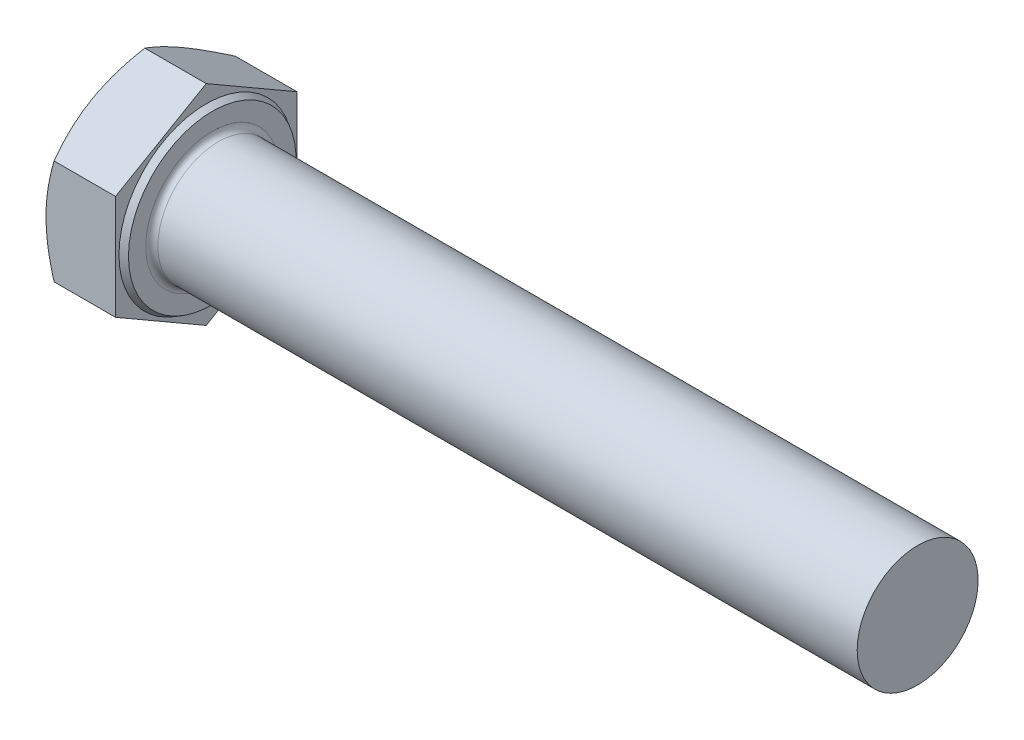
SolidWorks part; units mm, degrees
material "Q235"
ref_plane "Front Plane" through (0, 0, 0) normal (0, 0, 1) x (1, 0, 0)
ref_plane "Top Plane" through (0, 0, 0) normal (0, 1, 0) x (1, 0, 0)
ref_plane "Right Plane" through (0, 0, 0) normal (1, 0, 0) x (0, 0, -1)
sketch "Sketch1" plane through (0, 0, 0) normal (1, 0, 0) x (0, 0, -1)
  line L0 (9, 5.1962) -> (9, -5.1962)
  line L1 (-9, 5.1962) -> (-9, -5.1962)
  line L2 (9, -5.1962) -> (0, -10.3923)
  line L3 (0, -10.3923) -> (-9, -5.1962)
  line L4 (9, 5.1962) -> (0, 10.3923)
  line L5 (0, 10.3923) -> (-9, 5.1962)
  circle A0 centre (0, 0) radius 10.015 construction
  dimension "e" = 20.03
  dimension "s" = 18
  dimension "D2" = 120
  dimension "D3" = 9
  dimension "D4" = 9
  dimension "D5" = 9
extrude "Base-Extrude" add sketch "Sketch1" along normal blind 7.5
sketch "Sketch2" plane through (0, 0, 0) normal (0, 0, 1) x (1, 0, 0)
  line L0 (0, 5.1962) -> (0, -5.1962) construction
  line L1 (0, 0) -> (77.5, 0)
  line L2 (0, 0) -> (0, 6)
  line L3 (0, 6) -> (47.5, 6)
  line L4 (77.5, 0) -> (77.5, 4.4845)
  line L5 (7.5, 10.3923) -> (7.5, 5.1962) construction
  line L7 (0, 0) -> (89.5, 0) construction
  line L8 (77.5, -4.4845) -> (47.5, -6) construction
  line L9 (0, -6) -> (47.5, -6) construction
  line L10 (9.25, 6) -> (9.25, 0) construction
  line L11 (47.5, 15.24) -> (47.5, -1.27) construction
  line L12 (7.5, 5.1962) -> (7.5, -5.1962) construction
  line L13 (47.5, 6) -> (77.5, 6)
  line L14 (77.5, 6) -> (77.5, 4.4845)
  dimension "l" = 70
  dimension "d" = 12
  dimension "Minor_dia" = 8.969
  dimension "p" = 1.75
  dimension "b" = 30
  dimension "ds" = 12
revolve "Boss-Revolve1" add sketch "Sketch2" angle 360 about L7
cosmetic thread "Cosmetic Thread1" parameters "Thread_length"=30, "Thread_minor"=8.969
sketch "Sketch3" plane through (0, 0, 0) normal (0, 0, 1) x (1, 0, 0)
  line L0 (0, 9) -> (3.6906, 15.3923)
  line L1 (0, 10.3923) -> (0, 5.1962) construction
  line L2 (3.6906, 15.3923) -> (3.6906, 20.3923)
  line L3 (3.6906, 20.3923) -> (-10, 20.3923)
  line L4 (-10, 20.3923) -> (-10, 9)
  line L5 (-10, 9) -> (0, 9)
  line L6 (0, 0) -> (99.06, 0) construction
  line L7 (7.5, 10.3923) -> (0, 10.3923) construction
  dimension "D1" = 9
  dimension "D2" = 5
  dimension "D3" = 10
  dimension "D4" = 5
  dimension "Head_ch_ang" = 30
revolve "Cut-Revolve1" cut sketch "Sketch3" angle 360 about L6
sketch "Sketch4" plane through (0, 0, 0) normal (0, 0, 1) x (1, 0, 0)
  line L0 (7.5, 0) -> (7.5, 8.315) construction
  line L2 (7.5, -6) -> (7.5, 6) construction
  line L3 (7.5, 10.3923) -> (7.5, 5.1962) construction
  line L4 (7.5, 8.315) -> (6.9, 8.6614)
  line L5 (0, 0) -> (95.25, 0) construction
  line L6 (0, 0) -> (89.5, 0) construction
  line L9 (6.9, 8.6614) -> (6.9, 10.3923)
  line L10 (7.5, 10.3923) -> (0.8038, 10.3923) construction
  line L11 (6.9, 10.3923) -> (7.5, 10.3923)
  line L12 (7.5, 10.3923) -> (7.5, 8.315)
  dimension "D1" = 120
  dimension "c" = 0.6
  dimension "dw" = 16.63
revolve "Cut-Revolve3" cut sketch "Sketch4" angle 360 about L5
fillet "Fillet" radius 0.6 1 edges at (7.5, 0, -6)
sketch "Sketch6" plane through (0, 0, 0) normal (0, 0, 1) x (1, 0, 0)
  line L0 (0, 0) -> (77.5, 0) construction
  line L1 (77.5, -6) -> (77.5, 6) construction
  line L2 (77.5, 0) -> (77.5, 6) construction
  line L4 (76.625, 6) -> (78.375, 6)
  line L5 (76.625, 6) -> (77.5, 4.4845)
  line L6 (77.5, 4.4845) -> (78.375, 6)
  dimension "D1" = 1.75
revolve "Cut-Revolve4" [suppressed] cut sketch "Sketch6" angle 360 about L0
pattern_linear "LPattern1" [suppressed]
